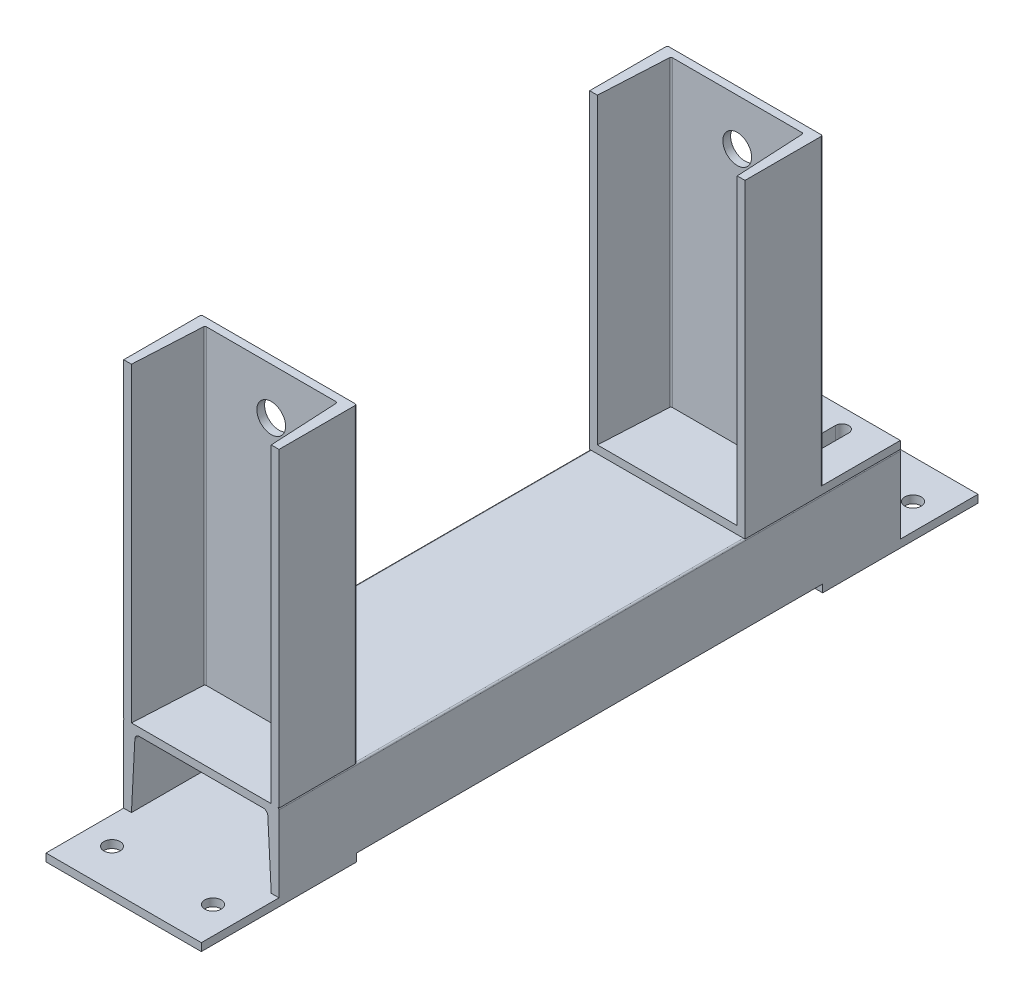
from build123d import *

# Parameters (mm, degrees)
BOSS_EXTRUDE1_DEPTH          = 400
SKETCH2_W                    = 100
SKETCH2_H                    = 100
BOSS_EXTRUDE2_DEPTH          = 5
F_10_5_10_5_DIAMETER_HOLE1_D = 10.5
BOSS_EXTRUDE3_DEPTH          = 200
SKETCH6_W                    = 100
SKETCH6_H                    = 100
BOSS_EXTRUDE4_DEPTH          = 5
BOSS_EXTRUDE5_DEPTH          = 195
CUT_EXTRUDE1_DEPTH           = 20
CUT_EXTRUDE1_DEPTH_BACK      = 20
F_18_5_18_5_DIAMETER_HOLE1_D = 18.5


with BuildPart() as part:
    # Sketch1 → Boss-Extrude1 (new body)
    with BuildSketch(Plane.XY):
        with BuildLine():
            Line((0, 0), (0, 49))
            ThreePointArc((0, 49), (0.292893219, 49.707106781), (1, 50))
            Line((1, 50), (99, 50))
            ThreePointArc((99, 50), (99.707106781, 49.707106781), (100, 49))
            Line((100, 49), (100, 0))
            Line((100, 0), (95, 0))
            Line((95, 0), (92.790644836, 42.157007869))
            ThreePointArc((92.790644836, 42.157007869), (91.859819959, 44.176123113), (89.794756232, 45))
            Line((89.794756232, 45), (10.205243768, 45))
            ThreePointArc((10.205243768, 45), (8.140180041, 44.176123113), (7.209355164, 42.157007869))
            Line((7.209355164, 42.157007869), (5, 0))
            Line((5, 0), (0, 0))
        make_face()
    extrude(amount=BOSS_EXTRUDE1_DEPTH)

    # Sketch2 → Boss-Extrude2 (add)
    with BuildSketch(Plane.XZ):
        with Locations((50, 400)):
            Rectangle(SKETCH2_W, SKETCH2_H)
        with Locations((50, 0)):
            Rectangle(SKETCH2_W, SKETCH2_H)
    extrude(amount=BOSS_EXTRUDE2_DEPTH)

    # Ø10.5 (10.5) Diameter Hole1 (through all)
    with Locations(Plane(origin=(0, 0, 0), x_dir=(1, 0, 0), z_dir=(0, 1, 0))):
        with Locations((17.5, -425), (82.5, -425), (83.148664141, 25), (17.5, 25)):
            Hole(F_10_5_10_5_DIAMETER_HOLE1_D / 2)

    # Sketch5 → Boss-Extrude3 (add)
    with BuildSketch(Plane(origin=(0, 50, 0), x_dir=(1, 0, 0), z_dir=(0, 1, 0))):
        with BuildLine():
            Line((1, -350), (99, -350))
            ThreePointArc((99, -350), (99.707106781, -350.292893219), (100, -351))
            Line((100, -351), (100, -400))
            Line((100, -400), (95, -400))
            Line((95, -400), (92.6913149, -355.947664044))
            ThreePointArc((92.6913149, -355.947664044), (92.381039941, -355.274625629), (91.692685366, -355))
            Line((91.692685366, -355), (8.307314634, -355))
            ThreePointArc((8.307314634, -355), (7.618960059, -355.274625629), (7.3086851, -355.947664044))
            Line((7.3086851, -355.947664044), (5, -400))
            Line((5, -400), (0, -400))
            Line((0, -400), (0, -351))
            ThreePointArc((0, -351), (0.292893219, -350.292893219), (1, -350))
        make_face()
    extrude(amount=BOSS_EXTRUDE3_DEPTH)

    # Sketch6 → Boss-Extrude4 (add)
    with BuildSketch(Plane(origin=(0, 50, 0), x_dir=(1, 0, 0), z_dir=(0, 1, 0))):
        with Locations((50, -50)):
            Rectangle(SKETCH6_W, SKETCH6_H)
    extrude(amount=BOSS_EXTRUDE4_DEPTH)

    # Sketch7 → Boss-Extrude5 (add)
    with BuildSketch(Plane(origin=(0, 55, 0), x_dir=(1, 0, 0), z_dir=(0, 1, 0))):
        with BuildLine():
            Line((1, -50), (99, -50))
            ThreePointArc((99, -50), (99.707106781, -50.292893219), (100, -51))
            Line((100, -51), (100, -100))
            Line((100, -100), (95, -100))
            Line((95, -100), (92.6913149, -55.947664044))
            ThreePointArc((92.6913149, -55.947664044), (92.381039941, -55.274625629), (91.692685366, -55))
            Line((91.692685366, -55), (8.307314634, -55))
            ThreePointArc((8.307314634, -55), (7.618960059, -55.274625629), (7.3086851, -55.947664044))
            Line((7.3086851, -55.947664044), (5, -100))
            Line((5, -100), (0, -100))
            Line((0, -100), (0, -51))
            ThreePointArc((0, -51), (0.292893219, -50.292893219), (1, -50))
        make_face()
    extrude(amount=BOSS_EXTRUDE5_DEPTH)

    # Sketch8 → Cut-Extrude1 (cut, two sides: drawn at the far end of the back side and taken through both)
    with BuildSketch(Plane(origin=(0, 50, 0), x_dir=(1, 0, 0), z_dir=(0, 1, 0)).offset(-CUT_EXTRUDE1_DEPTH_BACK)):
        with BuildLine():
            Line((20.75, -37.5), (20.75, -12.5))
            ThreePointArc((20.75, -12.5), (25, -8.25), (29.25, -12.5))
            Line((29.25, -12.5), (29.25, -37.5))
            ThreePointArc((29.25, -37.5), (25, -41.75), (20.75, -37.5))
        make_face()
        with BuildLine():
            Line((70.75, -37.5), (70.75, -12.5))
            ThreePointArc((70.75, -12.5), (75, -8.25), (79.25, -12.5))
            Line((79.25, -12.5), (79.25, -37.5))
            ThreePointArc((79.25, -37.5), (75, -41.75), (70.75, -37.5))
        make_face()
    extrude(amount=CUT_EXTRUDE1_DEPTH + CUT_EXTRUDE1_DEPTH_BACK, mode=Mode.SUBTRACT)

    # Ø18.5 (18.5) Diameter Hole1 (through all)
    with Locations(Plane(origin=(0, 0, 50), x_dir=(-1, 0, 0), z_dir=(0, 0, -1))):
        with Locations((-50, 220)):
            Hole(F_18_5_18_5_DIAMETER_HOLE1_D / 2)


solid = part.part
